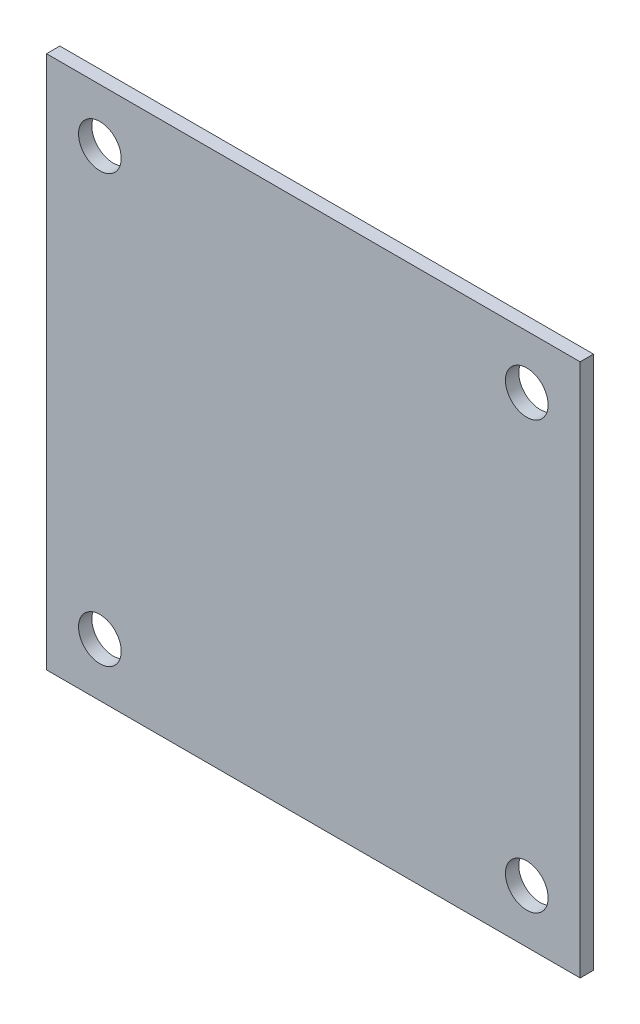
from build123d import *

# Parameters (mm, degrees)
SKETCH1_W           = 400
SKETCH1_H           = 400
SKETCH1_R           = 16
BOSS_EXTRUDE1_DEPTH = 10


with BuildPart() as part:
    # Sketch1 → Boss-Extrude1 (new body)
    with BuildSketch(Plane.XY):
        Rectangle(SKETCH1_W, SKETCH1_H)
        with Locations((-160, 160)):
            Circle(SKETCH1_R, mode=Mode.SUBTRACT)
        with Locations((160, 160)):
            Circle(SKETCH1_R, mode=Mode.SUBTRACT)
        with Locations((160, -160)):
            Circle(SKETCH1_R, mode=Mode.SUBTRACT)
        with Locations((-160, -160)):
            Circle(SKETCH1_R, mode=Mode.SUBTRACT)
    extrude(amount=BOSS_EXTRUDE1_DEPTH)


solid = part.part
